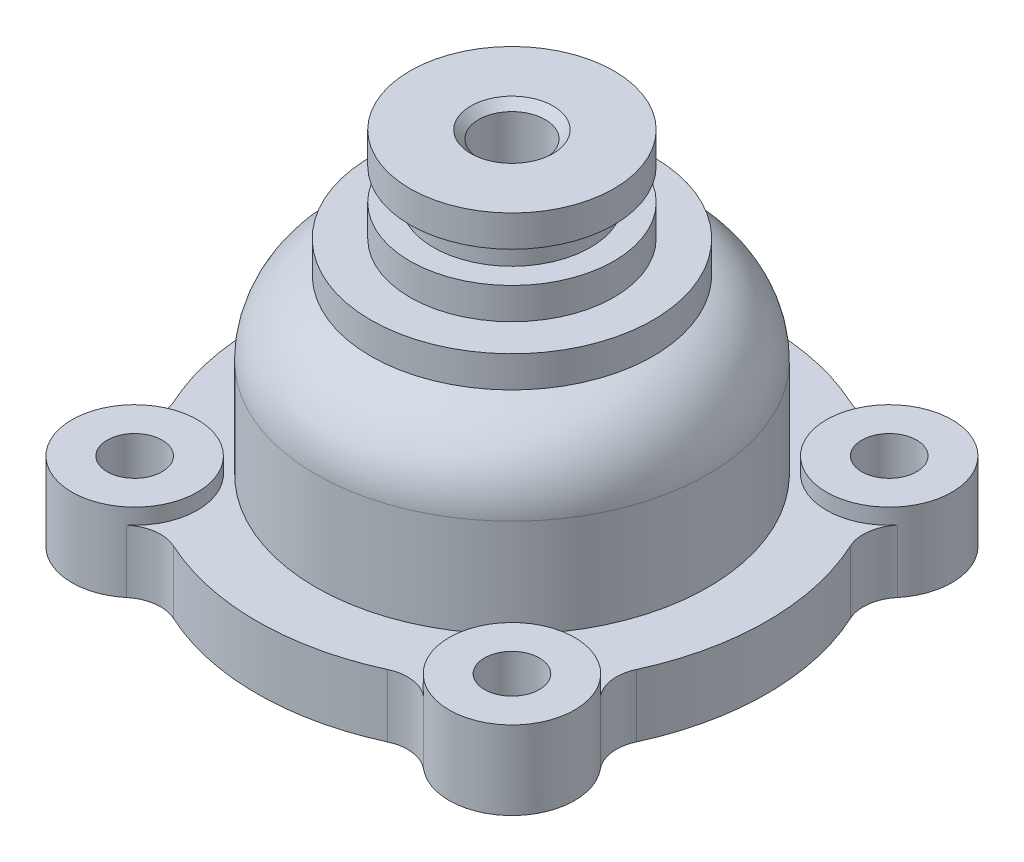
from build123d import *

# Parameters (mm, degrees)
M10_TAPPED_HOLE1_D  = 8.5
CHAMFER1_SIZE       = 1
SKETCH6_R           = 8
SKETCH6_R_2         = 3.5
BOSS_EXTRUDE1_DEPTH = 8
SKETCH7_R           = 3.5
CUT_EXTRUDE1_DEPTH  = 8
FILLET1_R           = 5
BOSS_EXTRUDE2_START = 2
SKETCH8_R           = 8
SKETCH8_R_2         = 3.5
BOSS_EXTRUDE2_DEPTH = 2


with BuildPart() as part:
    # Sketch1 → Revolve1 (revolve)
    with BuildSketch(Plane.XY, mode=Mode.PRIVATE) as revolve1_sk:
        with BuildLine():
            Line((0, 46), (-13, 46))
            Line((-13, 46), (-13, 42))
            Line((-13, 42), (-10, 42))
            Line((-10, 42), (-10, 38))
            Line((-10, 38), (-13, 38))
            Line((-13, 38), (-13, 34))
            Line((-13, 34), (-18, 34))
            Line((-18, 34), (-18, 30.006223624))
            ThreePointArc((-18, 30.006223624), (-23.062257748, 26.382911393), (-25, 20.46683161))
            Line((-25, 20.46683161), (-25, 8))
            Line((-25, 8), (-32.5, 8))
            Line((-32.5, 8), (-32.5, 0))
            Line((-32.5, 0), (-20, 0))
            Line((-20, 0), (-20, 21))
            ThreePointArc((-20, 21), (-18.535533906, 24.535533906), (-15, 26))
            Line((-15, 26), (0, 26))
            Line((0, 26), (0, 46))
        make_face()
    revolve(revolve1_sk.sketch.rotate(Axis((0, 0, 0), (0, 1, 0)), 270), axis=Axis((0, 0, 0), (0, 1, 0)))

    # M10 Tapped Hole1 (through all)
    with Locations(Plane(origin=(0, 46, 0), x_dir=(1, 0, 0), z_dir=(0, 1, 0))):
        with Locations((0, 0)):
            Hole(M10_TAPPED_HOLE1_D / 2)

    # Chamfer1
    chamfer1_edges = [part.edges().sort_by_distance(p)[0] for p in [
        (4.25, 46, 0),
    ]]
    chamfer(chamfer1_edges, length=CHAMFER1_SIZE)

    # Sketch6 → Boss-Extrude1 (add)
    # profile 1 of 4: a face of its own
    with BuildSketch(Plane(origin=(0, 8, 0), x_dir=(1, 0, 0), z_dir=(0, 1, 0))):
        with Locations((-24.04163056, 24.04163056)):
            Circle(SKETCH6_R)
        with Locations((-24.04163056, 24.04163056)):
            Circle(SKETCH6_R_2, mode=Mode.SUBTRACT)
    # profile 2 of 4: a face of its own
    with BuildSketch(Plane(origin=(0, 8, 0), x_dir=(1, 0, 0), z_dir=(0, 1, 0))):
        with Locations((24.04163056, 24.04163056)):
            Circle(SKETCH6_R)
        with Locations((24.04163056, 24.04163056)):
            Circle(SKETCH6_R_2, mode=Mode.SUBTRACT)
    # profile 3 of 4: a face of its own
    with BuildSketch(Plane(origin=(0, 8, 0), x_dir=(1, 0, 0), z_dir=(0, 1, 0))):
        with Locations((24.04163056, -24.04163056)):
            Circle(SKETCH6_R)
        with Locations((24.04163056, -24.04163056)):
            Circle(SKETCH6_R_2, mode=Mode.SUBTRACT)
    # profile 4 of 4: a face of its own
    with BuildSketch(Plane(origin=(0, 8, 0), x_dir=(1, 0, 0), z_dir=(0, 1, 0))):
        with Locations((-24.04163056, -24.04163056)):
            Circle(SKETCH6_R)
        with Locations((-24.04163056, -24.04163056)):
            Circle(SKETCH6_R_2, mode=Mode.SUBTRACT)
    extrude(amount=-BOSS_EXTRUDE1_DEPTH)

    # Sketch7 → Cut-Extrude1 (cut)
    with BuildSketch(Plane(origin=(0, 8, 0), x_dir=(1, 0, 0), z_dir=(0, 1, 0))):
        with Locations(Location((-24.04163056, 24.04163056, 0), (0, 0, 270))):
            Circle(SKETCH7_R)
        with Locations(Location((24.04163056, 24.04163056, 0), (0, 0, 270))):
            Circle(SKETCH7_R)
        with Locations(Location((24.04163056, -24.04163056, 0), (0, 0, 270))):
            Circle(SKETCH7_R)
        with Locations(Location((-24.04163056, -24.04163056, 0), (0, 0, 270))):
            Circle(SKETCH7_R)
    extrude(amount=-CUT_EXTRUDE1_DEPTH, mode=Mode.SUBTRACT)

    # Fillet1
    fillet1_edges = [part.edges().sort_by_distance(p)[0] for p in [
        (-16.944361965, 4, -27.733348113),
        (-27.733348113, 4, -16.944361965),
        (-27.733348113, 4, 16.944361965),
        (-16.944361965, 4, 27.733348113),
        (16.944361965, 4, 27.733348113),
        (27.733348113, 4, 16.944361965),
        (27.733348113, 4, -16.944361965),
        (16.944361965, 4, -27.733348113),
    ]]
    fillet(fillet1_edges, radius=FILLET1_R)

    # Sketch8 → Boss-Extrude2 (add)
    # profile 1 of 4: a face of its own
    with BuildSketch(Plane(origin=(0, 8, 0), x_dir=(1, 0, 0), z_dir=(0, 1, 0)).offset(BOSS_EXTRUDE2_START)):
        with Locations(Location((-24.04163056, 24.04163056, 0), (0, 0, 270))):
            Circle(SKETCH8_R)
        with Locations(Location((-24.04163056, 24.04163056, 0), (0, 0, 270))):
            Circle(SKETCH8_R_2, mode=Mode.SUBTRACT)
    # profile 2 of 4: a face of its own
    with BuildSketch(Plane(origin=(0, 8, 0), x_dir=(1, 0, 0), z_dir=(0, 1, 0)).offset(BOSS_EXTRUDE2_START)):
        with Locations(Location((24.04163056, 24.04163056, 0), (0, 0, 270))):
            Circle(SKETCH8_R)
        with Locations(Location((24.04163056, 24.04163056, 0), (0, 0, 270))):
            Circle(SKETCH8_R_2, mode=Mode.SUBTRACT)
    # profile 3 of 4: a face of its own
    with BuildSketch(Plane(origin=(0, 8, 0), x_dir=(1, 0, 0), z_dir=(0, 1, 0)).offset(BOSS_EXTRUDE2_START)):
        with Locations(Location((24.04163056, -24.04163056, 0), (0, 0, 270))):
            Circle(SKETCH8_R)
        with Locations(Location((24.04163056, -24.04163056, 0), (0, 0, 270))):
            Circle(SKETCH8_R_2, mode=Mode.SUBTRACT)
    # profile 4 of 4: a face of its own
    with BuildSketch(Plane(origin=(0, 8, 0), x_dir=(1, 0, 0), z_dir=(0, 1, 0)).offset(BOSS_EXTRUDE2_START)):
        with Locations(Location((-24.04163056, -24.04163056, 0), (0, 0, 270))):
            Circle(SKETCH8_R)
        with Locations(Location((-24.04163056, -24.04163056, 0), (0, 0, 270))):
            Circle(SKETCH8_R_2, mode=Mode.SUBTRACT)
    extrude(amount=-BOSS_EXTRUDE2_DEPTH)


solid = part.part
